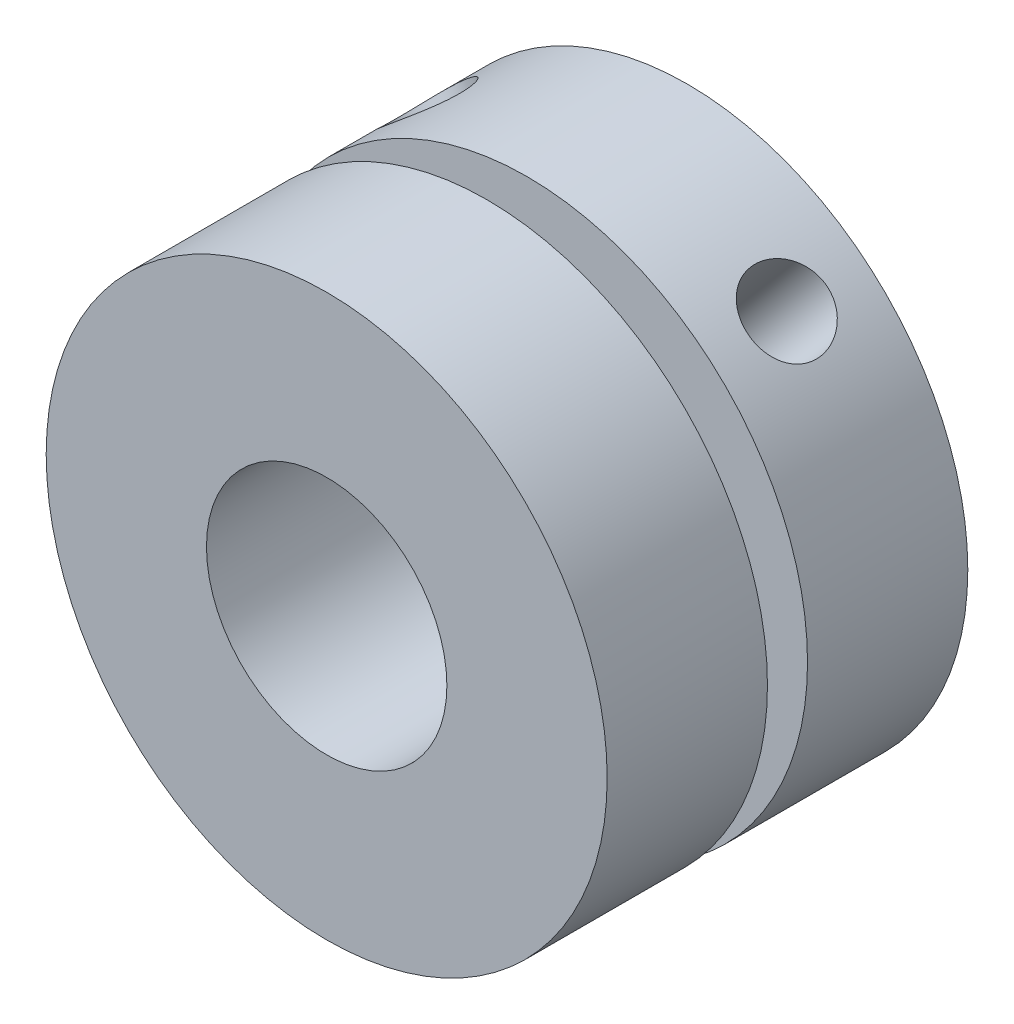
from build123d import *

# Parameters (mm, degrees)
SKETCH1_R           = 35
SKETCH1_R_2         = 15
BOSS_EXTRUDE1_DEPTH = 20
SKETCH2_R           = 20
SKETCH2_R_2         = 15
BOSS_EXTRUDE2_DEPTH = 5
BOSS_EXTRUDE3_START = 20
SKETCH5_R           = 35
BOSS_EXTRUDE3_DEPTH = 20
BOSS_EXTRUDE4_START = 10
SKETCH6_R           = 20
BOSS_EXTRUDE4_DEPTH = 10


with BuildPart() as part:
    # Sketch1 → Boss-Extrude1 (new body)
    with BuildSketch(Plane.XY):
        Circle(SKETCH1_R)
        Circle(SKETCH1_R_2, mode=Mode.SUBTRACT)
    extrude(amount=BOSS_EXTRUDE1_DEPTH)

    # Sketch2 → Boss-Extrude2 (add, symmetric)
    with BuildSketch(Plane(origin=(0, 0, 0), x_dir=(-1, 0, 0), z_dir=(0, 0, -1))):
        with Locations(Location((0, 0, 0), (0, 0, 180))):
            Circle(SKETCH2_R)
        Circle(SKETCH2_R_2, mode=Mode.SUBTRACT)
    extrude(amount=BOSS_EXTRUDE2_DEPTH, both=True)

    # Sketch5 → Boss-Extrude3 (add)
    with BuildSketch(Plane(origin=(0, 0, -5), x_dir=(-1, 0, 0), z_dir=(0, 0, -1)).offset(BOSS_EXTRUDE3_START)):
        with Locations(Location((0, 0, 0), (0, 0, 180))):
            Circle(SKETCH5_R)
    extrude(amount=-BOSS_EXTRUDE3_DEPTH)

    # Sketch6 → Boss-Extrude4 (add)
    with BuildSketch(Plane(origin=(0, 0, -25), x_dir=(-1, 0, 0), z_dir=(0, 0, -1)).offset(BOSS_EXTRUDE4_START)):
        with Locations(Location((0, 0, 0), (0, 0, 180))):
            Circle(SKETCH6_R)
    extrude(amount=-BOSS_EXTRUDE4_DEPTH)

    # Sketch11 → Cut-Revolve2 (revolve, cut)
    with BuildSketch(Plane.XY.offset(-15)):
        Polygon((-11.623419421, 13.852251853), (-23.246838841, 27.704503705), (-19.416616626, 30.918441754), (-7.793197205, 17.066189901), align=None)
    revolve(axis=Axis((-11.623419421, 13.852251853, -15), (-0.642787609686535, 0.7660444431189817, 0)), mode=Mode.SUBTRACT)

    # Sketch17 → Cut-Revolve3 (revolve, cut)
    with BuildSketch(Plane.XY.offset(-15)):
        Polygon((12.450815126, 14.838303658), (24.416664753, 29.098647939), (28.246886969, 25.88470989), (16.281037342, 11.624365609), align=None)
    revolve(axis=Axis((12.450815126, 14.838303658, -15), (0.6427876096865406, 0.766044443118977, 0)), mode=Mode.SUBTRACT)


solid = part.part
